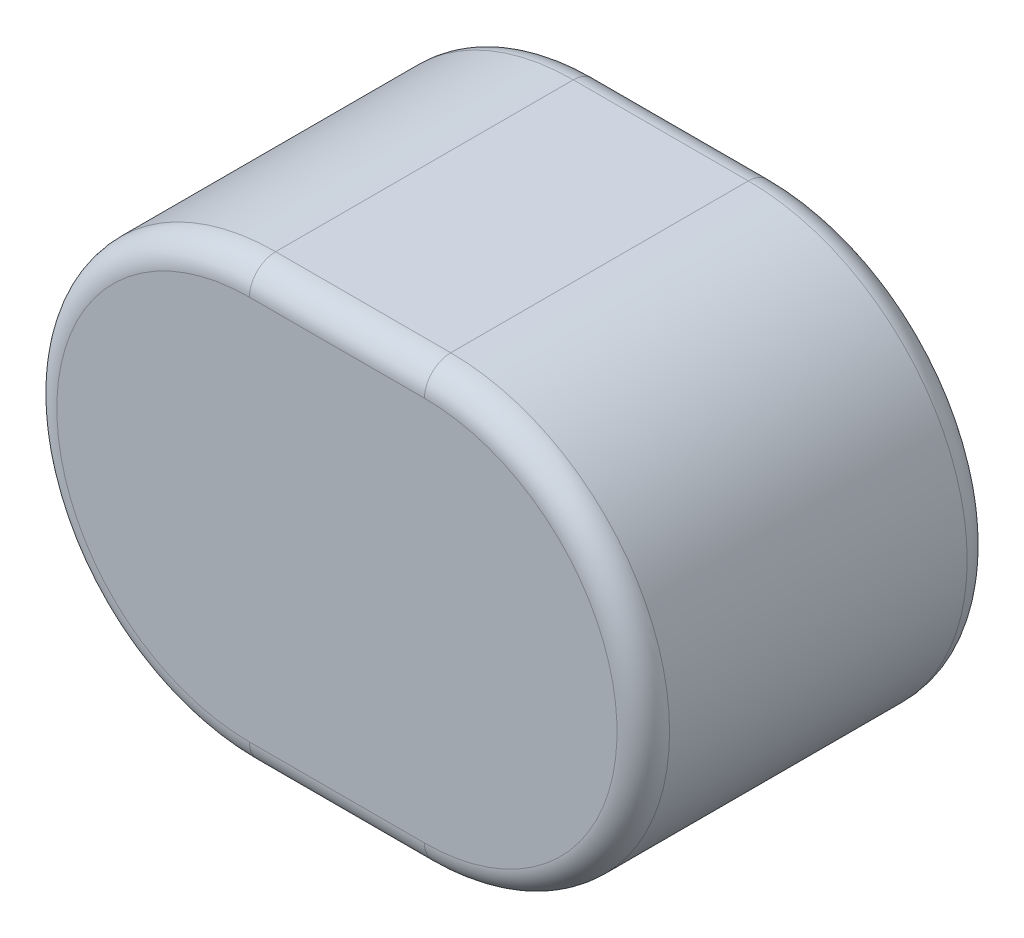
SolidWorks part; units mm, degrees
material "45"
ref_plane "基准面1" through (0, 0, 0) normal (0, 0, 1) x (1, 0, 0)
ref_plane "基准面2" through (0, 0, 0) normal (0, 1, 0) x (1, 0, 0)
ref_plane "基准面3" through (0, 0, 0) normal (1, 0, 0) x (0, 0, -1)
sketch "尺寸草图" plane through (0, 0, 0) normal (0, 0, 1) x (1, 0, 0)
  line L0 (-7, 0) -> (7, 0) construction
  point P3 (-8, 0)
  point P4 (-0.6, 0)
  point P5 (0, 0)
  point P8 (-10, 0)
  point P11 (0, 0)
sketch "草图1" plane through (0, 0, 0) normal (0, 0, 1) x (1, 0, 0)
  line L0 (-28.0599, 0) -> (30.562, 0) construction
  line L1 (-2, 5) -> (2, 5)
  line L2 (-2, -5) -> (2, -5)
  line L3 (0, 2.9108) -> (0, -2.1805) construction
  arc A0 (-2, 5) -> (-2, -5) centre (-2, 0) ccw
  arc A1 (2, 5) -> (2, -5) centre (2, 0) cw
extrude "基体-拉伸" add sketch "草图1" along normal blind 8
fillet "圆角1" radius 0.6 8 edges at (7, 0, 8) (0, 5, 8) (-7, 0, 8) (0, 5, 0) (7, 0, 0) (0, -5, 0) (-7, 0, 0) (0, -5, 8)
equation "\"D3@草图1\" = \"L@尺寸草图\""
equation "\"D1@草图1\" = \"b@尺寸草图\" / 2"
equation "\"D1@圆角1\" = \"r@尺寸草图\""
equation "\"D1@基体-拉伸\" = \"h@尺寸草图\""
